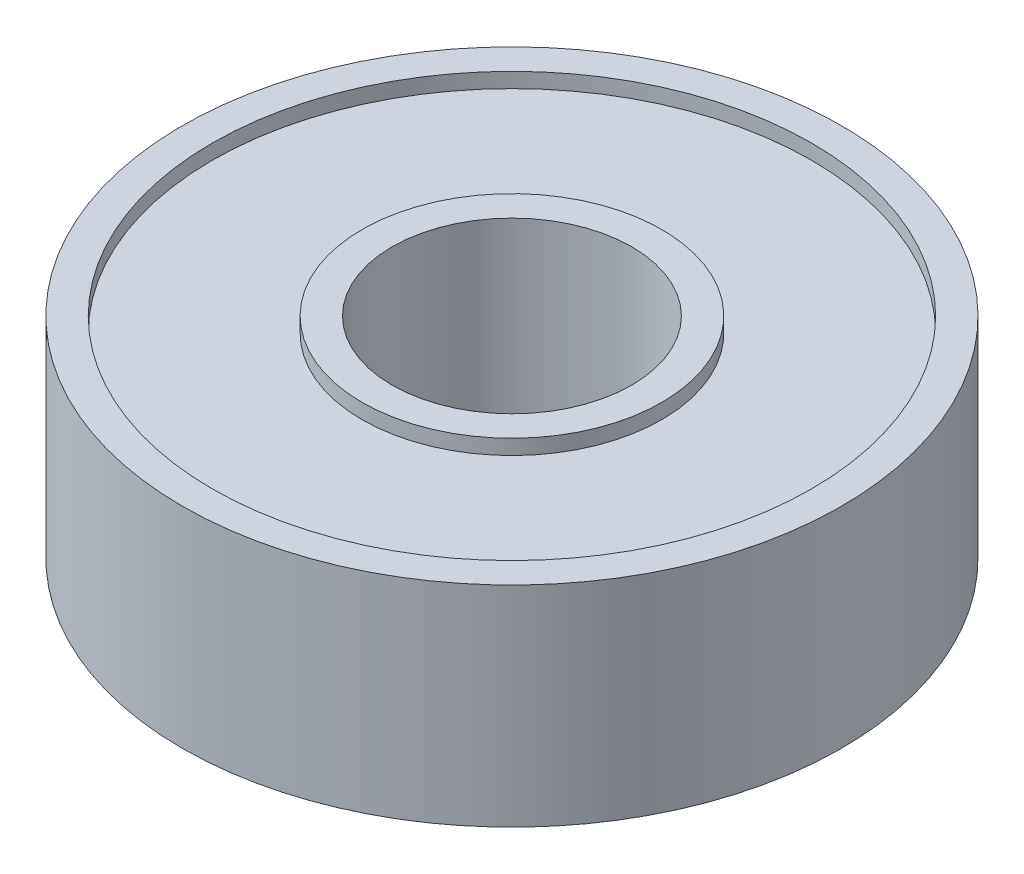
from build123d import *

# Parameters (mm, degrees)
SKETCH1_R           = 11
SKETCH1_R_2         = 4
BOSS_EXTRUDE1_DEPTH = 7
SKETCH2_R           = 10
SKETCH2_R_2         = 5
CUT_EXTRUDE1_DEPTH  = 0.5
CUT_EXTRUDE2_START  = -0.5
SKETCH3_R           = 10
SKETCH3_R_2         = 5
CUT_EXTRUDE2_DEPTH  = 0.5


with BuildPart() as part:
    # Sketch1 → Boss-Extrude1 (new body)
    with BuildSketch(Plane(origin=(0, 0, 0), x_dir=(1, 0, 0), z_dir=(0, 1, 0))):
        with Locations(Location((0, 0, 0), (0, 0, 270))):
            Circle(SKETCH1_R)
        with Locations(Location((0, 0, 0), (0, 0, 270))):
            Circle(SKETCH1_R_2, mode=Mode.SUBTRACT)
    extrude(amount=BOSS_EXTRUDE1_DEPTH)

    # Sketch2 → Cut-Extrude1 (cut)
    with BuildSketch(Plane.XZ):
        with Locations(Location((0, 0, 0), (0, 0, 270))):
            Circle(SKETCH2_R)
        with Locations(Location((0, 0, 0), (0, 0, 270))):
            Circle(SKETCH2_R_2, mode=Mode.SUBTRACT)
    extrude(amount=-CUT_EXTRUDE1_DEPTH, mode=Mode.SUBTRACT)

    # Sketch3 → Cut-Extrude2 (cut)
    with BuildSketch(Plane(origin=(0, 7, 0), x_dir=(1, 0, 0), z_dir=(0, 1, 0)).offset(CUT_EXTRUDE2_START)):
        with Locations(Location((0, 0, 0), (0, 0, 90))):
            Circle(SKETCH3_R)
        with Locations(Location((0, 0, 0), (0, 0, 90))):
            Circle(SKETCH3_R_2, mode=Mode.SUBTRACT)
    extrude(amount=CUT_EXTRUDE2_DEPTH, mode=Mode.SUBTRACT)


solid = part.part
